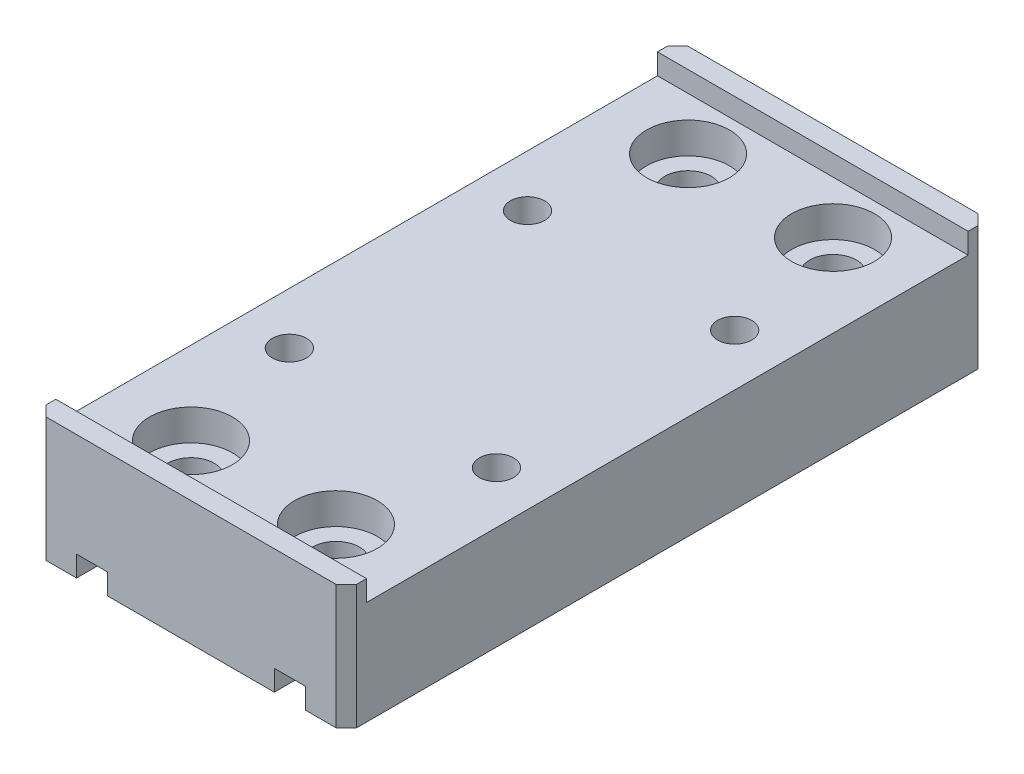
SolidWorks part; units mm, degrees
ref_plane "前视基准面" through (0, 0, 0) normal (0, 0, 1) x (1, 0, 0)
ref_plane "上视基准面" through (0, 0, 0) normal (0, 1, 0) x (1, 0, 0)
ref_plane "右视基准面" through (0, 0, 0) normal (1, 0, 0) x (0, 0, -1)
sketch "草图1" plane through (0, 0, 0) normal (0, 1, 0) x (1, 0, 0)
  line L1 (-15, 31) -> (15, 31)
  line L2 (-15, 31) -> (-15, -31)
  line L3 (-15, -31) -> (15, -31)
  line L4 (15, 31) -> (15, -31)
  line L5 (-15, 31) -> (15, -31) construction
  line L6 (-15, -31) -> (15, 31) construction
  point P0 (0, 0)
  dimension "D1" = 30
  dimension "D2" = 62
extrude "凸台-拉伸1" add sketch "草图1" along normal blind 12
sketch "草图2" plane through (0, 0, 0) normal (0, -1, 0) x (1, 0, 0)
  line L1 (-11.05, 28.05) -> (11.05, 28.05)
  line L2 (-11.05, 28.05) -> (-11.05, -28.05)
  line L3 (-11.05, -28.05) -> (11.05, -28.05)
  line L4 (11.05, 28.05) -> (11.05, -28.05)
  line L5 (-11.05, 28.05) -> (11.05, -28.05) construction
  line L6 (-11.05, -28.05) -> (11.05, 28.05) construction
  point P0 (0, 0)
  dimension "D1" = 22.1
  dimension "D2" = 56.1
extrude "切除-拉伸1" cut sketch "草图2" against normal blind 2
sketch "草图3" plane through (0, 0, 0) normal (0, -1, 0) x (1, 0, 0)
  line L0 (-11.05, 28.05) -> (-11.05, -28.05) construction
  line L1 (-8.05, 36.8263) -> (-11.05, 36.8263)
  line L2 (-8.05, 36.8263) -> (-8.05, -35.3129)
  line L3 (-8.05, -35.3129) -> (-11.05, -35.3129)
  line L4 (-11.05, 36.8263) -> (-11.05, -35.3129)
  line L5 (-8.05, 36.8263) -> (-11.05, -35.3129) construction
  line L6 (-8.05, -35.3129) -> (-11.05, 36.8263) construction
  point P0 (-9.55, 0.7567)
  dimension "D1" = 3
extrude "切除-拉伸2" cut sketch "草图3" against normal blind 2
mirror "镜向1" about plane through (0, 0, 0) normal (1, 0, 0) of "切除-拉伸2"
sketch "草图4" plane through (0, 12, 0) normal (0, 1, 0) x (1, 0, 0)
  line L1 (-43.0463, 29.05) -> (43.0463, 29.05)
  line L2 (-43.0463, 29.05) -> (-43.0463, -29.05)
  line L3 (-43.0463, -29.05) -> (43.0463, -29.05)
  line L4 (43.0463, 29.05) -> (43.0463, -29.05)
  line L5 (-43.0463, 29.05) -> (43.0463, -29.05) construction
  line L6 (-43.0463, -29.05) -> (43.0463, 29.05) construction
  point P0 (0, 0)
  dimension "D1" = 58.1
extrude "切除-拉伸3" cut sketch "草图4" against normal blind 2
hole_wizard "M4 螺纹孔1" positions "草图6" profile "草图5" tap size "M4" standard "GB" end condition through all
sketch "草图6" plane through (0, 10, 0) normal (0, 1, 0) x (1, 0, 0)
  line L0 (-10, 11.5) -> (-10, -11.5) construction
  line L3 (0, 0) -> (-10, 0) construction
  line L7 (-15, 29.05) -> (-15, -29.05) construction
  point P0 (-10, 11.5)
  point P2 (10, 11.5)
  point P4 (-10, -11.5)
  point P6 (10, -11.5)
  dimension "D1" = 5
  dimension "D2" = 23
  dimension "D3" = 20
sketch "草图5" plane through (-10, 10, -11.5) normal (1, 0, 0) x (0, 0, 1)
  line L0 (0, 0) -> (0, 10)
  line L1 (0, 10) -> (1.65, 10)
  line L2 (1.65, 10) -> (1.65, 0)
  line L5 (1.65, 0) -> (0, 0)
  line L11 (0, -6.35) -> (0, 107.95) construction
  dimension "通孔螺纹孔钻头直径" = 3.3
  dimension "通孔螺纹孔钻头深度" = 10
cosmetic thread "孔螺蚊线1" parameters "D2"=4
cosmetic thread "孔螺蚊线2" parameters "D2"=4
cosmetic thread "孔螺蚊线3" parameters "D2"=4
cosmetic thread "孔螺蚊线4" parameters "D2"=4
hole_wizard "打孔尺寸(%根据)开槽圆柱头螺钉的类型1" positions "草图8" profile "草图7" counterbore size "M4" standard "GB" end condition through all
sketch "草图8" plane through (0, 12, 0) normal (0, 1, 0) x (1, 0, 0)
  line L0 (-7, 24) -> (7, 24) construction
  line L1 (7, 24) -> (7, -24) construction
  line L4 (0, 0) -> (0, 24) construction
  line L7 (0, 0) -> (7, 0) construction
  point P0 (-7, 24)
  point P2 (7, 24)
  point P4 (-7, -24)
  point P6 (7, -24)
  dimension "D1" = 14
  dimension "D2" = 48
sketch "草图7" plane through (-7, 12, -24) normal (1, 0, 0) x (0, 0, 1)
  line L0 (0, 0) -> (0, 12)
  line L1 (0, 12) -> (2.25, 12)
  line L3 (2.25, 12) -> (2.25, 5)
  line L4 (2.25, 5) -> (4, 5)
  line L5 (4, 5) -> (4, 0)
  line L7 (4, 0) -> (0, 0)
  line L11 (0, -6.35) -> (0, 107.95) construction
  dimension "通孔孔直径" = 4.5
  dimension "通孔孔深度" = 12
  dimension "柱形沉头孔直径" = 8
  dimension "柱形沉头孔深度" = 5
chamfer "倒角1" distance 1 angle 45 4 edges at (-15, 6, -31) (15, 6, -31) (-15, 6, 31) (15, 6, 31)
